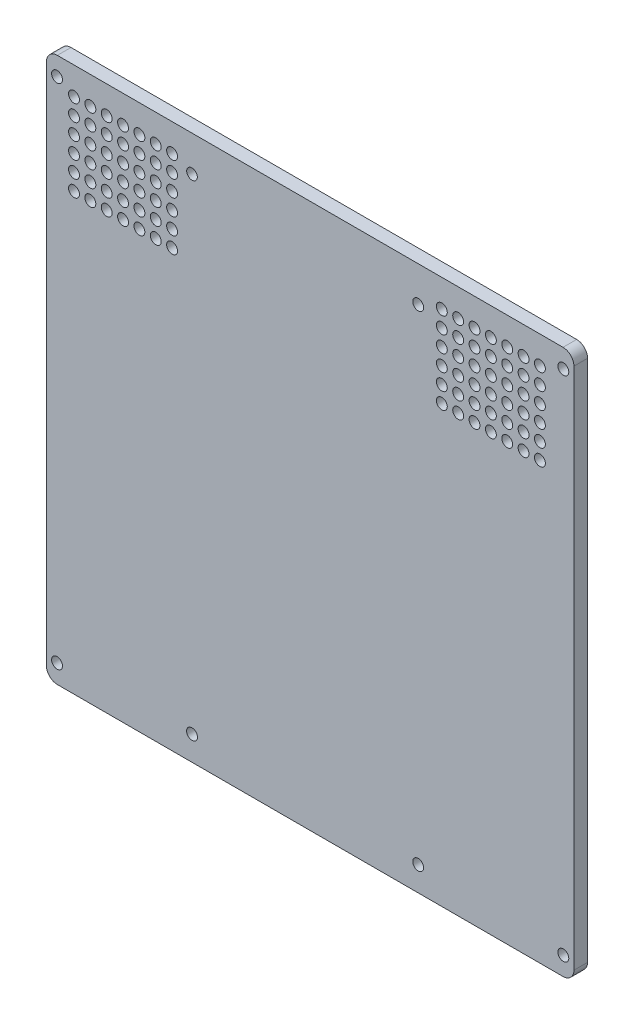
from build123d import *

# Parameters (mm, degrees)
SKETCH1_W           = 193.6
SKETCH1_H           = 200
BOSS_EXTRUDE1_DEPTH = 5
SKETCH3_R           = 2
SKETCH3_R_2         = 1.952382978
CUT_EXTRUDE2_DEPTH  = 12
SKETCH4_R           = 2
CUT_EXTRUDE3_DEPTH  = 10
FILLET1_R           = 4
SKETCH5_R           = 2
CUT_EXTRUDE4_DEPTH  = 10
LPATTERN1_COUNT     = 2
LPATTERN1_PITCH     = 135


with BuildPart() as part:
    # Sketch1 → Boss-Extrude1 (new body)
    with BuildSketch(Plane.XY):
        with Locations((58.2, -87.878787879)):
            Rectangle(SKETCH1_W, SKETCH1_H)
    extrude(amount=BOSS_EXTRUDE1_DEPTH)

    # Sketch3 → Cut-Extrude2 (cut)
    with BuildSketch(Plane.XY.offset(5)):
        with Locations((97.841313089, -178.911029975)):
            Circle(SKETCH3_R)
        with Locations((97.841313089, -0.892985434)):
            Circle(SKETCH3_R)
        with Locations((14.826966281, -178.911029975)):
            Circle(SKETCH3_R)
        with Locations((14.826966281, -0.892985434)):
            Circle(SKETCH3_R_2)
    extrude(amount=-CUT_EXTRUDE2_DEPTH, mode=Mode.SUBTRACT)

    # Sketch4 → Cut-Extrude3 (cut)
    with BuildSketch(Plane.XY.offset(5)):
        with Locations((151.109433088, -181.043069679)):
            Circle(SKETCH4_R)
        with Locations((151.109433088, 5.285493921)):
            Circle(SKETCH4_R)
        with Locations((-34.709433088, 5.285493921)):
            Circle(SKETCH4_R)
        with Locations((-34.709433088, -181.043069679)):
            Circle(SKETCH4_R)
    extrude(amount=-CUT_EXTRUDE3_DEPTH, mode=Mode.SUBTRACT)

    # Fillet1
    fillet1_edges = [part.edges().sort_by_distance(p)[0] for p in [
        (-38.6, 12.121212121, 2.5),
        (155, 12.121212121, 2.5),
        (155, -187.878787879, 2.5),
        (-38.6, -187.878787879, 2.5),
    ]]
    fillet(fillet1_edges, radius=FILLET1_R)

    # Sketch5 → Cut-Extrude4 (cut)
    with BuildSketch(Plane.XY.offset(5)):
        with Locations((142.515403652, 1.981764562)):
            Circle(SKETCH5_R)
        with Locations((136.515403652, 1.981764562)):
            Circle(SKETCH5_R)
        with Locations((130.515403652, 1.981764562)):
            Circle(SKETCH5_R)
        with Locations((124.515403652, 1.981764562)):
            Circle(SKETCH5_R)
        with Locations((118.515403652, 1.981764562)):
            Circle(SKETCH5_R)
        with Locations((112.515403652, 1.981764562)):
            Circle(SKETCH5_R)
        with Locations((106.515403652, 1.981764562)):
            Circle(SKETCH5_R)
        with Locations((136.515403652, -4.018235438)):
            Circle(SKETCH5_R)
        with Locations((130.515403652, -4.018235438)):
            Circle(SKETCH5_R)
        with Locations((124.515403652, -4.018235438)):
            Circle(SKETCH5_R)
        with Locations((118.515403652, -4.018235438)):
            Circle(SKETCH5_R)
        with Locations((112.515403652, -4.018235438)):
            Circle(SKETCH5_R)
        with Locations((106.515403652, -4.018235438)):
            Circle(SKETCH5_R)
        with Locations((136.515403652, -10.018235438)):
            Circle(SKETCH5_R)
        with Locations((130.515403652, -10.018235438)):
            Circle(SKETCH5_R)
        with Locations((124.515403652, -10.018235438)):
            Circle(SKETCH5_R)
        with Locations((118.515403652, -10.018235438)):
            Circle(SKETCH5_R)
        with Locations((112.515403652, -10.018235438)):
            Circle(SKETCH5_R)
        with Locations((106.515403652, -10.018235438)):
            Circle(SKETCH5_R)
        with Locations((136.515403652, -16.018235438)):
            Circle(SKETCH5_R)
        with Locations((130.515403652, -16.018235438)):
            Circle(SKETCH5_R)
        with Locations((124.515403652, -16.018235438)):
            Circle(SKETCH5_R)
        with Locations((118.515403652, -16.018235438)):
            Circle(SKETCH5_R)
        with Locations((112.515403652, -16.018235438)):
            Circle(SKETCH5_R)
        with Locations((106.515403652, -16.018235438)):
            Circle(SKETCH5_R)
        with Locations((136.515403652, -22.018235438)):
            Circle(SKETCH5_R)
        with Locations((130.515403652, -22.018235438)):
            Circle(SKETCH5_R)
        with Locations((124.515403652, -22.018235438)):
            Circle(SKETCH5_R)
        with Locations((118.515403652, -22.018235438)):
            Circle(SKETCH5_R)
        with Locations((112.515403652, -22.018235438)):
            Circle(SKETCH5_R)
        with Locations((106.515403652, -22.018235438)):
            Circle(SKETCH5_R)
        with Locations((136.515403652, -28.018235438)):
            Circle(SKETCH5_R)
        with Locations((130.515403652, -28.018235438)):
            Circle(SKETCH5_R)
        with Locations((124.515403652, -28.018235438)):
            Circle(SKETCH5_R)
        with Locations((118.515403652, -28.018235438)):
            Circle(SKETCH5_R)
        with Locations((112.515403652, -28.018235438)):
            Circle(SKETCH5_R)
        with Locations((106.515403652, -28.018235438)):
            Circle(SKETCH5_R)
        with Locations((142.515403652, -4.018235438)):
            Circle(SKETCH5_R)
        with Locations((142.515403652, -10.018235438)):
            Circle(SKETCH5_R)
        with Locations((142.515403652, -16.018235438)):
            Circle(SKETCH5_R)
        with Locations((142.515403652, -22.018235438)):
            Circle(SKETCH5_R)
        with Locations((142.515403652, -28.018235438)):
            Circle(SKETCH5_R)
    cut_extrude4 = extrude(amount=-CUT_EXTRUDE4_DEPTH, mode=Mode.SUBTRACT)

    # LPattern1: Cut-Extrude4 ×2
    with Locations(*[(-i * LPATTERN1_PITCH, 0, 0) for i in range(1, LPATTERN1_COUNT)]):
        add(cut_extrude4, mode=Mode.SUBTRACT)


solid = part.part
